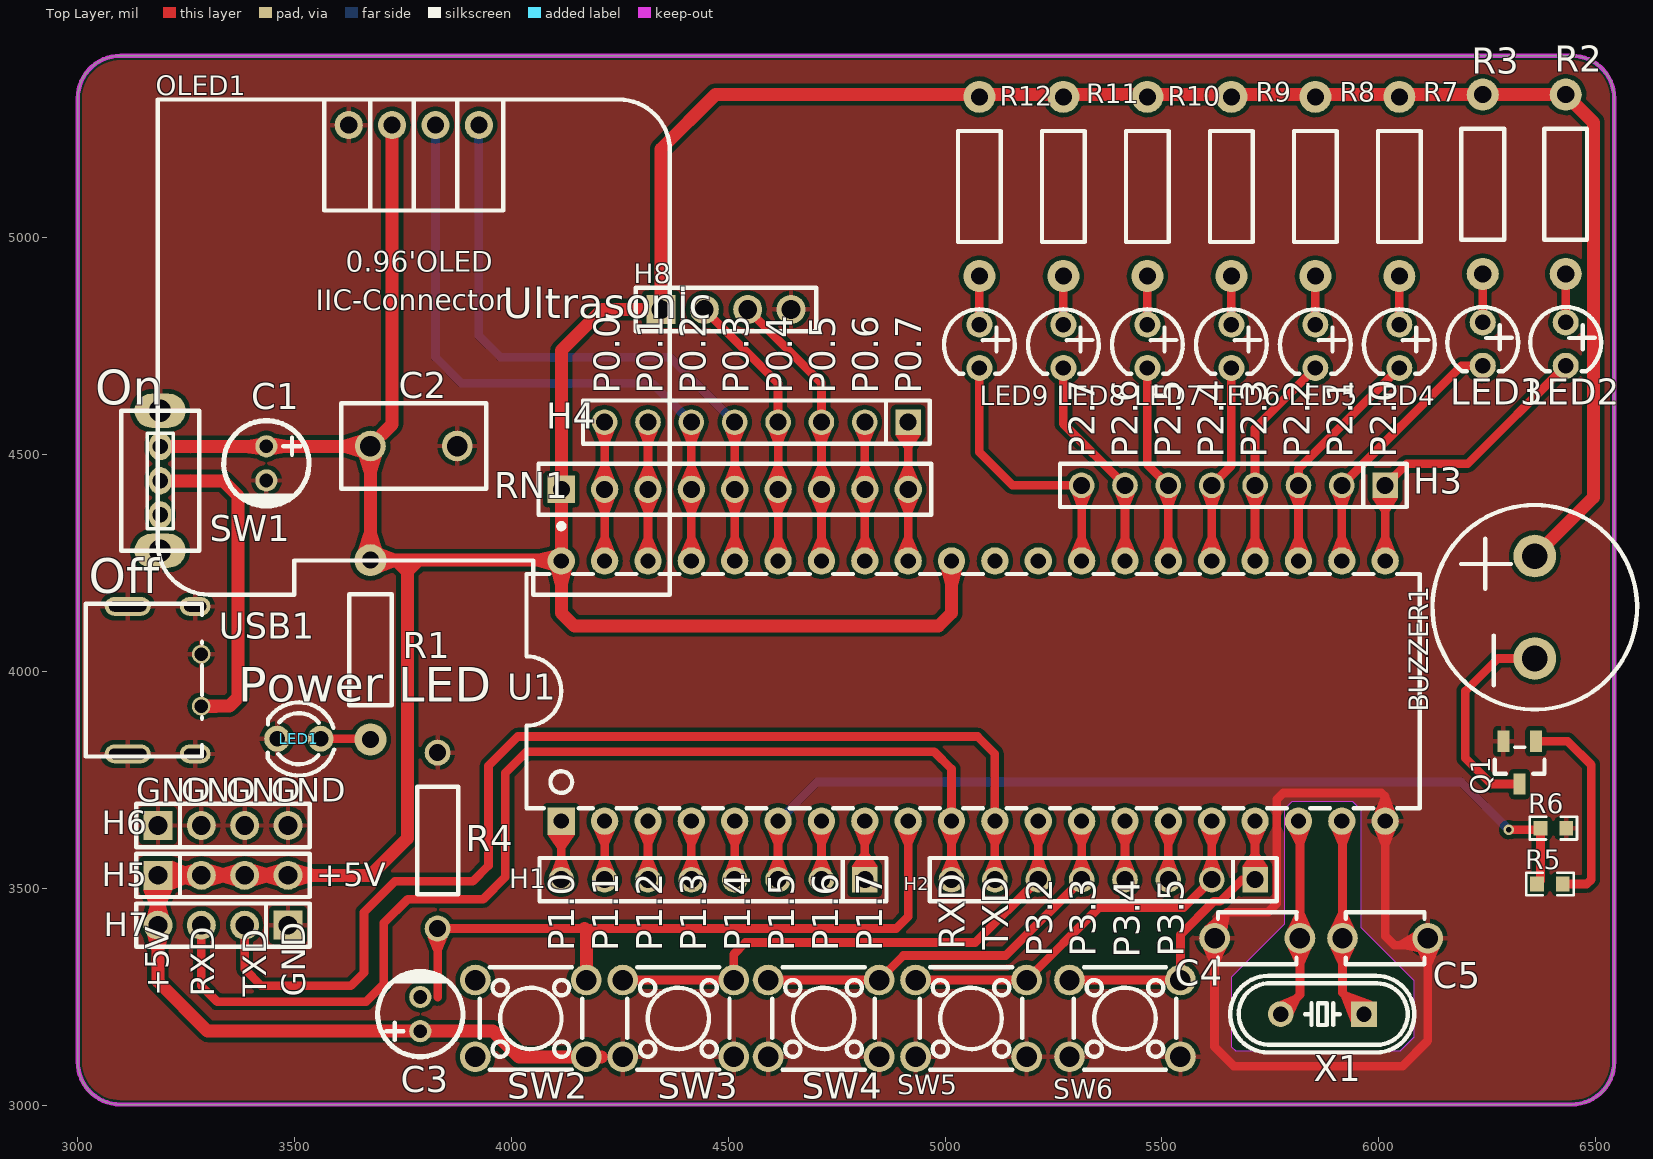
[diagram p0: Top Layer view]
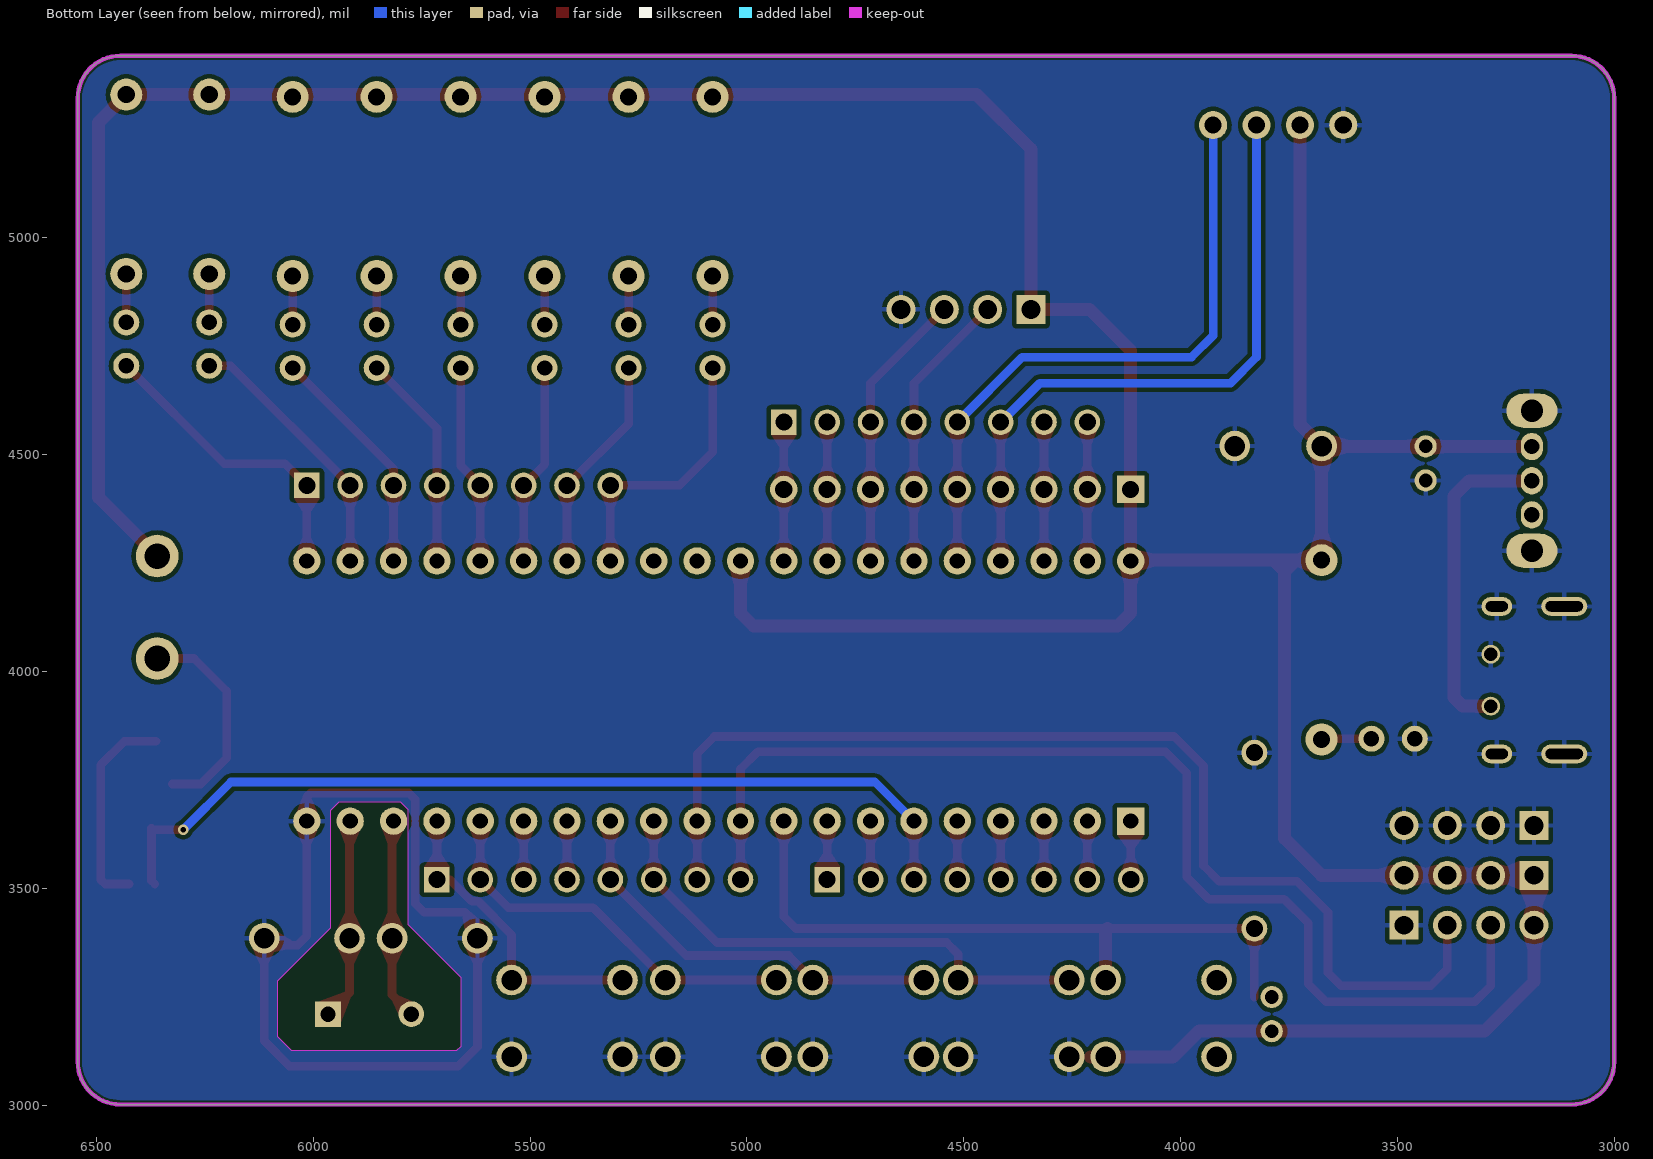
[diagram p1: Bottom Layer view, seen from below]
# Altium PCB MISC49889.pcbdoc
Units mil, origin at the board's own origin, x right, y up, seen from the top; angles counter-clockwise.
Board outline 3543.31 x 2418.5 mil, 2 copper layers (Top Layer, Bottom Layer), stack 62.206 mil thick; 47 components, 49 nets, 191 pads, 1 vias.

## Layer stack, top to bottom
Top Solder Mask Layer: solder mask 0.394, Dk 3.3
Top Layer: signal copper 1.379
Dielectric1: surface 59.449, FR4, Dk 4.5
Bottom Layer: signal copper 1.378
Bottom Solder Mask Layer: solder mask 0.394, Dk 3.3

## Board outline
3098.43,5420 ccw(c3098.43,5321.57) 3000,5321.57 3000,3099.92 ccw(c3098.43,3099.92) 3098.43,3001.5 6444.88,3001.5 ccw(c6444.88,3099.92) 6543.31,3099.92 6543.31,5321.57 ccw(c6444.88,5321.57) 6444.88,5420 3098.43,5420

## Design rules (kind name [scope] priority, off if disabled: settings)
BoardOutlineClearance copperThickness2oz_1 [All] p2 off: genericclearance=8 ignorepadtopadclearanceinfootprint=FALSE except(0: Arc-SplitContinuation Track-SplitContinuation SMDPad-SplitContinuation THPad-SplitContinuation Via-SplitContinuation Fill-SplitContinuation Region-SplitContinuation Poly-SplitContinuation Text-SplitContinuation Hole-SplitContinuation; 6: SMDPad-CutoutEdge THPad-CutoutEdge Via-CutoutEdge Fill-CutoutEdge Region-CutoutEdge Text-CutoutEdge Hole-CutoutEdge; 10: Poly-OutlineEdge Poly-CutoutEdge; 11.8: Arc-OutlineEdge Track-OutlineEdge SMDPad-OutlineEdge THPad-OutlineEdge Via-OutlineEdge Fill-OutlineEdge Region-OutlineEdge Text-OutlineEdge Hole-OutlineEdge Arc-CutoutEdge Track-CutoutEdge)
BoardOutlineClearance Plane_innerPlane_1 [All] p4 off: genericclearance=6 ignorepadtopadclearanceinfootprint=FALSE except(0: Arc-SplitContinuation Track-SplitContinuation SMDPad-SplitContinuation THPad-SplitContinuation Via-SplitContinuation Fill-SplitContinuation Region-SplitContinuation Poly-SplitContinuation Text-SplitContinuation Hole-SplitContinuation; 5.98: SMDPad-CutoutEdge THPad-CutoutEdge Via-CutoutEdge Fill-CutoutEdge Region-CutoutEdge Text-CutoutEdge Hole-CutoutEdge; 10: Poly-OutlineEdge Poly-CutoutEdge; 11.81: Arc-OutlineEdge Track-OutlineEdge SMDPad-OutlineEdge THPad-OutlineEdge Via-OutlineEdge Fill-OutlineEdge Region-OutlineEdge Text-OutlineEdge Hole-OutlineEdge Arc-CutoutEdge Track-CutoutEdge)
BoardOutlineClearance Copper_copperRegion_1 [All] p6 off: genericclearance=6 ignorepadtopadclearanceinfootprint=FALSE except(0: Arc-SplitContinuation Track-SplitContinuation SMDPad-SplitContinuation THPad-SplitContinuation Via-SplitContinuation Fill-SplitContinuation Region-SplitContinuation Poly-SplitContinuation Text-SplitContinuation Hole-SplitContinuation; 5.98: SMDPad-CutoutEdge THPad-CutoutEdge Via-CutoutEdge Fill-CutoutEdge Region-CutoutEdge Text-CutoutEdge Hole-CutoutEdge; 10: Poly-OutlineEdge Poly-CutoutEdge; 11.81: Arc-OutlineEdge Track-OutlineEdge SMDPad-OutlineEdge THPad-OutlineEdge Via-OutlineEdge Fill-OutlineEdge Region-OutlineEdge Text-OutlineEdge Hole-OutlineEdge Arc-CutoutEdge Track-CutoutEdge)
BoardOutlineClearance copperThickness1oz_1 [All] p8: genericclearance=6 ignorepadtopadclearanceinfootprint=FALSE except(0: Arc-SplitContinuation Track-SplitContinuation SMDPad-SplitContinuation THPad-SplitContinuation Via-SplitContinuation Fill-SplitContinuation Region-SplitContinuation Poly-SplitContinuation Text-SplitContinuation Hole-SplitContinuation; 5.98: SMDPad-CutoutEdge THPad-CutoutEdge Via-CutoutEdge Fill-CutoutEdge Region-CutoutEdge Text-CutoutEdge Hole-CutoutEdge; 10: Poly-OutlineEdge Poly-CutoutEdge; 11.81: Arc-OutlineEdge Track-OutlineEdge SMDPad-OutlineEdge THPad-OutlineEdge Via-OutlineEdge Fill-OutlineEdge Region-OutlineEdge Text-OutlineEdge Hole-OutlineEdge Arc-CutoutEdge Track-CutoutEdge)
Clearance copperThickness2oz [All] p1 off: gap=8 ignorepadtopadclearanceinfootprint=FALSE except(6: SMDPad-Track SMDPad-SMDPad THPad-Track SMDPad-THPad THPad-THPad Track-Via SMDPad-Via THPad-Via Via-Via Fill-Track Region-Track Fill-SMDPad Region-SMDPad Fill-THPad Region-THPad Fill-Via Region-Via Fill-Fill Fill-Region Region-Region Arc-Track Arc-SMDPad Arc-THPad Arc-Via Fill-Arc Region-Arc Arc-Arc Text-Track SMDPad-Text Text-THPad Text-Via Fill-Text Region-Text Arc-Text Text-Text Hole-Track Hole-SMDPad Hole-THPad Hole-Via Fill-Hole Region-Hole Hole-Arc Hole-Text; 10: Poly-Track Poly-SMDPad Poly-THPad Poly-Via Poly-Fill Poly-Region Poly-Poly Poly-Arc Poly-Text Poly-Hole)
Clearance Plane_innerPlane [All] p3 off: gap=6 ignorepadtopadclearanceinfootprint=FALSE except(5.98: SMDPad-Track SMDPad-SMDPad THPad-Track SMDPad-THPad THPad-THPad Track-Via SMDPad-Via THPad-Via Via-Via Fill-Track Region-Track Fill-SMDPad Region-SMDPad Fill-THPad Region-THPad Fill-Via Region-Via Fill-Fill Fill-Region Region-Region Arc-Track Arc-SMDPad Arc-THPad Arc-Via Fill-Arc Region-Arc Arc-Arc Text-Track SMDPad-Text Text-THPad Text-Via Fill-Text Region-Text Arc-Text Text-Text Hole-Track Hole-SMDPad Hole-THPad Hole-Via Fill-Hole Region-Hole Hole-Arc Hole-Text; 10: Poly-Track Poly-SMDPad Poly-THPad Poly-Via Poly-Fill Poly-Region Poly-Poly Poly-Arc Poly-Text Poly-Hole)
Clearance Copper_copperRegion [All] p5 off: gap=6 ignorepadtopadclearanceinfootprint=FALSE except(5.98: SMDPad-Track SMDPad-SMDPad THPad-Track SMDPad-THPad THPad-THPad Track-Via SMDPad-Via THPad-Via Via-Via Fill-Track Region-Track Fill-SMDPad Region-SMDPad Fill-THPad Region-THPad Fill-Via Region-Via Fill-Fill Fill-Region Region-Region Arc-Track Arc-SMDPad Arc-THPad Arc-Via Fill-Arc Region-Arc Arc-Arc Text-Track SMDPad-Text Text-THPad Text-Via Fill-Text Region-Text Arc-Text Text-Text Hole-Track Hole-SMDPad Hole-THPad Hole-Via Fill-Hole Region-Hole Hole-Arc Hole-Text; 10: Poly-Track Poly-SMDPad Poly-THPad Poly-Via Poly-Fill Poly-Region Poly-Poly Poly-Arc Poly-Text Poly-Hole)
Clearance copperThickness1oz [All] p7: gap=6 ignorepadtopadclearanceinfootprint=FALSE except(5.98: SMDPad-Track SMDPad-SMDPad THPad-Track SMDPad-THPad THPad-THPad Track-Via SMDPad-Via THPad-Via Via-Via Fill-Track Region-Track Fill-SMDPad Region-SMDPad Fill-THPad Region-THPad Fill-Via Region-Via Fill-Fill Fill-Region Region-Region Arc-Track Arc-SMDPad Arc-THPad Arc-Via Fill-Arc Region-Arc Arc-Arc Text-Track SMDPad-Text Text-THPad Text-Via Fill-Text Region-Text Arc-Text Text-Text Hole-Track Hole-SMDPad Hole-THPad Hole-Via Fill-Hole Region-Hole Hole-Arc Hole-Text; 10: Poly-Track Poly-SMDPad Poly-THPad Poly-Via Poly-Fill Poly-Region Poly-Poly Poly-Arc Poly-Text Poly-Hole)
DiffPairsRouting differentialPair [All] p1: maxlimit=6 minlimit=6 mostfreqgap=6 toplayer_minwidth=5 toplayer_prefwidth=10 toplayer_maxwidth=100 toplayer_mingap=6 toplayer_prefgap=6 toplayer_maxgap=6 bottomlayer_minwidth=5 bottomlayer_prefwidth=10 bottomlayer_maxwidth=100 bottomlayer_mingap=6 bottomlayer_prefgap=6 bottomlayer_maxgap=6 maxuncoupledlength=10
HoleToHoleClearance otherClearance [All] p1: gap=11.8 allowstackedmicrovias=TRUE
Length netLength [All] p1: minlimit=0 maxlimit=0
PasteMaskExpansion pasteMaskExpansion [All] p1: expansion=0
PlaneConnect innerPlane [All] p1: planeconnectstyle=Relief reliefexpansion=20 reliefentries=4 reliefconductorwidth=10 reliefairgap=10
PolygonConnect copperRegion [All] p1: connectstyle=Relief reliefconductorwidth=10 reliefentries=4 polygonreliefangle="90 Angle" airgapwidth=10 via.connectstyle=Relief via.reliefconductorwidth=10 via.reliefentries=4 via.polygonreliefangle="90 Angle" via.airgapwidth=10
RoutingVias viaSize [All] p1: holewidth=12 width=24 viastyle="Through Hole" minholewidth=11.8 minwidth=19.7 maxholewidth=248 maxwidth=393.7
SolderMaskExpansion solderMaskExpansion [IsVia] p1: expansion=-1000 istentingtop=TRUE
SolderMaskExpansion solderMaskExpansion [All] p2: expansion=2 istentingtop=FALSE
Width copperThickness2oz_2 [All] p1 off: maxlimit=100 minlimit=8 preferedwidth=10
Width copperThickness1oz_2 [All] p2: maxlimit=100 minlimit=5 preferedwidth=10

## Components (designator, comment, footprint, x,y, rotation, side; value= is the part's Value field where it differs from the comment)
BUZZER1 "buzzer" BUZ-TH_BD12.0-P6.00-D0.9-RD 6360.02,4148.07 r90 top
C1 "10uF" CAP-TH_BD5.0-P2.00-D0.8-FD 3435,4480 r270 top
C2 "100nF" CAP-TH_L8.5-W5.0-P5.00-D1.2 3775,4520 r180 top
C3 "10uF" CAP-TH_BD5.0-P2.00-D0.8-FD 3790,3210 r90 top
C4 "47pF" CAP-TH_L4.5-W3.0-P5.00-D1.2 5720,3385 r0 top
C5 "47pF" CAP-TH_L4.5-W3.0-P5.00-D1.2 6015,3385 r180 top
H1 "" HDR-TH_8P-P2.54-V-M 4465,3520 r180 top
H2 "" HDR-TH_8P-P2.54-V-M 5365,3520 r180 top
H3 "" HDR-TH_8P-P2.54-V-M 5665,4429.22 r180 top
H4 "" HDR-TH_8P-P2.54-V-M 4565,4575 r180 top
H5 "" HDR-TH_4P-P2.54-V-M 3335,3530 r0 top
H6 "" HDR-TH_4P-P2.54-V-M 3335,3645 r0 top
H7 "" HDR-TH_4P-P2.54-V-M 3335,3415 r180 top
H8 "" HDR-TH_4P-P2.54-V-F 4495,4835 r0 top
LED1 "204-10SURD/S530-A3-L" LED-TH_BD3.0-P2.54-FD 3510,3845 r180 top
LED2 "204-10SYGD/S530-E3" LED-TH_BD3.8-P2.54-FD 6431.32,4755 r270 top
LED3 "204-10SYGD/S530-E3" LED-TH_BD3.8-P2.54-FD 6240,4755 r270 top
LED4 "204-10SYGD/S530-E3" LED-TH_BD3.8-P2.54-FD 6047.65,4750 r270 top
LED5 "204-10SYGD/S530-E3" LED-TH_BD3.8-P2.54-FD 5853.97,4750 r270 top
LED6 "204-10SYGD/S530-E3" LED-TH_BD3.8-P2.54-FD 5660.3,4750 r270 top
LED7 "204-10SYGD/S530-E3" LED-TH_BD3.8-P2.54-FD 5466.62,4750 r270 top
LED8 "204-10SYGD/S530-E3" LED-TH_BD3.8-P2.54-FD 5272.95,4750 r270 top
LED9 "204-10SYGD/S530-E3" LED-TH_BD3.8-P2.54-FD 5079.27,4750 r270 top
OLED1 "" 0.96OLED_4P 3775,5260 r0 top
Q1 "" S8550P_SOT 6325.02,3787.99 r90 top
R1 "1kΩ" RES-TH_BD2.5-L6.5-P10.50-D0.6 3675,4050 r270 top
R2 "1kΩ" RES-TH_BD2.5-L6.5-P10.50-D0.6 6431.32,5123.52 r270 top
R3 "1kΩ" RES-TH_BD2.5-L6.5-P10.50-D0.6 6240,5123.52 r270 top
R4 "10kΩ" RES-TH_BD2.4-L6.3-P10.30-D0.6 3830,3610 r270 top
R5 "1K" R0603 6395,3510 r0 top
R6 "1K" R0603 6402.72,3638.61 r0 top
R7 "1kΩ" RES-TH_BD2.5-L6.5-P10.50-D0.6 6047.65,5118.52 r270 top
R8 "1kΩ" RES-TH_BD2.5-L6.5-P10.50-D0.6 5853.97,5118.52 r270 top
R9 "1kΩ" RES-TH_BD2.5-L6.5-P10.50-D0.6 5660.3,5118.52 r270 top
R10 "1kΩ" RES-TH_BD2.5-L6.5-P10.50-D0.6 5466.62,5118.52 r270 top
R11 "1kΩ" RES-TH_BD2.5-L6.5-P10.50-D0.6 5272.95,5118.52 r270 top
R12 "1kΩ" RES-TH_BD2.5-L6.5-P10.50-D0.6 5079.27,5118.52 r270 top
RN1 "10kΩ" RES-ARRAY-TH_9P-P2.54-D1.0 4515.15,4420.16 r0 top
SW1 "SS-12D02-VG4" SW-TH_SS-12D02-VG4 3190,4440 r90 top
SW2 "" SW-TH_4P-L6.0-W6.0-P4.50-LS6.5 4045,3200 r180 top
SW3 "" SW-TH_4P-L6.0-W6.0-P4.50-LS6.5 4385,3200 r0 top
SW4 "" SW-TH_4P-L6.0-W6.0-P4.50-LS6.5 4720,3200 r0 top
SW5 "" SW-TH_4P-L6.0-W6.0-P4.50-LS6.5 5060,3200 r0 top
SW6 "" SW-TH_4P-L6.0-W6.0-P4.50-LS6.5 5415,3200 r0 top
U1 "STC89C52RC-40I-PDIP40" DIP-40_L52.0-W13.7-P2.54-LS15.2-BL 5065,3955 r0 top
USB1 "TYPE-C-31-M-33" USB-C-TH_TYPE-C-31-M-33 3200,3980 r270 top
X1 "11.0592MHz" HC-49US_L11.5-W4.5-P4.88 5870,3210 r180 top

## Footprints (in the part's own frame and the unit in brackets; to place one, negate y for a bottom-side part, rotate by r counter-clockwise, add the part's x,y. Pads: shape width x height; smd on the part's side, far side on the other; paste and mask are expansions set on the pad)
0.96OLED_4P [mm]
  round 1.65 hole 1 copper offset 0,0: 1(-3.81,-0.001) 2(-1.27,0.002) 3(1.27,0.002) 4(3.81,0.002)
  silkscreen extent -15,-27.5 15,1.5
BUZ-TH_BD12.0-P6.00-D0.9-RD [mm]
  round 2.5 hole 1.5 paste+0 mask+0.05: 1(-3,0) 2(3,0)
  silkscreen extent -5.99,-5.99 5.99,5.99
CAP-TH_BD5.0-P2.00-D0.8-FD [mm]
  round 1.3 hole 0.8 paste+0 mask+0.051: 1(-1,0) 2(1,0)
  silkscreen extent -2.5,-2.5 2.5,2.5
CAP-TH_L4.5-W3.0-P5.00-D1.2 [mm]
  round 1.8 hole 1.2 paste+0 mask+0.051: 1(-2.5,0) 2(2.5,0)
  silkscreen extent -2.3,-1.52 2.31,1.52
CAP-TH_L8.5-W5.0-P5.00-D1.2 [mm]
  round 1.8 hole 1.2 paste+0 mask+0.051: 1(-2.54,0) 2(2.54,0)
  silkscreen extent -4.25,-2.5 4.25,2.5
DIP-40_L52.0-W13.7-P2.54-LS15.2-BL [mil]
  rect 63x63 hole 35 paste+0 mask+2: 1(-950,-300)
  round 63 hole 35 paste+0 mask+2: 2(-850,-300) 3(-750,-300) 4(-650,-300) 5(-550,-300) 6(-450,-300) 7(-350,-300) 8(-250,-300) 9(-150,-300) 10(-50,-300) 11(50,-300) 12(150,-300) 13(250,-300) 14(350,-300) 15(450,-300) 16(550,-300) 17(650,-300) 18(750,-300) 19(850,-300) 20(950,-300) 21(950,300) 22(850,300) 23(750,300) 24(650,300) 25(550,300) 26(450,300) 27(350,300) 28(250,300) 29(150,300) 30(50,300) 31(-50,300) 32(-150,300) 33(-250,300) 34(-350,300) 35(-450,300) 36(-550,300) 37(-650,300) 38(-750,300) 39(-850,300) 40(-950,300)
  silkscreen extent -1030,-270 1030,270
HC-49US_L11.5-W4.5-P4.88 [mm]
  rect 1.5x1.5 hole 0.9 paste+0 mask+0.051: 1(-2.44,0)
  round 1.5 hole 0.9 paste+0 mask+0.051: 2(2.44,0)
  silkscreen extent -5.39,-2.25 5.39,2.25
HDR-TH_4P-P2.54-V-F [mm]
  rect 1.7x1.7 hole 1.1: 1(-3.81,0)
  round 1.7 hole 1.1: 2(-1.27,0) 3(1.27,0) 4(3.81,0)
  silkscreen extent -5.29,-1.27 5.29,1.27
HDR-TH_4P-P2.54-V-M [mm]
  rect 1.7x1.7 hole 1.1 paste+0 mask+0.051: 1(-3.81,0)
  round 1.7 hole 1.1 paste+0 mask+0.051: 2(-1.27,0) 3(1.27,0) 4(3.81,0)
  silkscreen extent -5.08,-1.27 5.08,1.27
HDR-TH_8P-P2.54-V-M [mm]
  rect 1.5x1.5 hole 1 paste+0 mask+0.051: 1(-8.89,0)
  round 1.5 hole 1 paste+0 mask+0.051: 2(-6.35,0) 3(-3.81,0) 4(-1.27,0) 5(1.27,0) 6(3.81,0) 7(6.35,0) 8(8.89,0)
  silkscreen extent -10.16,-1.27 10.16,1.27
LED-TH_BD3.0-P2.54-FD [mil]
  round 60 hole 36 paste+0 mask+2: 1(-50,0) 2(50,0)
  silkscreen extent -81,-84 72,85
LED-TH_BD3.8-P2.54-FD [mil]
  round 60 hole 35.43 paste+0 mask+2: 1(-50,0) 2(50,0)
  silkscreen extent -85,-82 63,82
R0603 [mil]
  rect 31.75x34.02 smd paste-3937.01 mask+2: 1(-29.66,0) 2(29.66,0)
  silkscreen extent -55,-26 55,26
RES-ARRAY-TH_9P-P2.54-D1.0 [mm]
  rect 1.6x1.6 hole 1 paste+0 mask+0.051: 1(-10.16,0)
  round 1.6 hole 1 paste+0 mask+0.051: 2(-7.62,0) 3(-5.08,0) 4(-2.54,0) 5(0,0) 6(2.54,0) 7(5.08,0) 8(7.62,0) 9(10.16,0)
  silkscreen extent -11.5,-2.31 11.5,1.5
RES-TH_BD2.4-L6.3-P10.30-D0.6 [mil]
  round 60 hole 39.37 paste+0 mask+2: 1(-202.76,0) 2(202.76,0)
  silkscreen extent -124,-47 124,47
RES-TH_BD2.5-L6.5-P10.50-D0.6 [mil]
  round 74 hole 39.37 paste+0 mask+2: 1(-206.69,0) 2(206.69,0)
  silkscreen extent -128,-49 128,49
S8550P_SOT [mil]
  rect 49.2x27.6 smd paste+0 mask+2: 1(50.84,-37.4) 2(50.84,37.4) 3(-47.56,0)
  silkscreen extent -24,-58 37,58
SW-TH_4P-L6.0-W6.0-P4.50-LS6.5 [mm]
  round 1.8 hole 1.2 paste+0 mask+0.051: 1(-3.25,2.25) 2(3.25,2.25) 3(-3.25,-2.25) 4(3.25,-2.25)
  silkscreen extent -3,-3 3,3
SW-TH_SS-12D02-VG4 [mm]
  oval 1.6x1.3 hole 0.9 paste+0 mask+0.051: 1(-2,0) 2(-0.007,0) 3(2,0)
  oval 2x3 hole 1.3 paste+0 mask+0.051: 4(4.1,0) 5(-4.1,0)
  silkscreen extent -4.1,-2.29 4.1,2.29
USB-C-TH_TYPE-C-31-M-33 [mm]
  oval 1.1x1.8 hole 0.6 slot 1.3 at 90 deg paste+0 mask+0.05: 3(4.32,1.8) 6(-4.32,1.8)
  oval 1.1x2.7 hole 0.6 slot 2.2 at 90 deg paste+0 mask+0.05: 4(4.32,-2.15) 5(-4.32,-2.15)
  round 1.1 hole 0.8 paste+0 mask+0.05: A9(1.52,2.15) B12(-1.52,2.15)
  silkscreen extent -4.47,-4.6 4.47,2.2

## Via types
v1: diameter 24, hole 12, Top Layer to Bottom Layer, 1 vias

## Nets (pads, with @x,y where several pads share a name; then routed paths per layer and width w, separated by ;. In a path a pad name is that pad's centre, name@x,y a point inside that pad or via, vN(x,y) a via of type N, cw(c..) or ccw(c..) an arc to the next point about the centre after c; other vN are vias at no path point)
$1N2977: LED1.1 R1.2 | length 120.7
  Top Layer w20: LED1.1 3678.31,3845 R1.2@3680,3843.31
$1N4098: LED2.1 R2.2 | length 111.8
  Top Layer w20: LED2.1 R2.2
$1N4101: LED3.1 R3.2 | length 111.8
  Top Layer w20: LED3.1 R3.2
$1N15801: Q1.1 R5.2 | length 484.4
  Top Layer w20: Q1.1 6436.17,3838.83 6490,3785 6490,3520 6480,3510 R5.2
$1N15923: BUZZER1.1 Q1.3 | length 495.8
  Top Layer w20: Q1.3 6259.57,3740.43 6200,3800 6200,3955 6274.96,4029.96 BUZZER1.1
$1N16102: LED5.1 R8.2 | length 111.8
  Top Layer w20: LED5.1 R8.2
$1N16108: LED4.1 R7.2 | length 111.8
  Top Layer w20: LED4.1 R7.2
$1N16243: LED7.1 R10.2 | length 111.8
  Top Layer w20: LED7.1 R10.2
$1N16249: LED6.1 R9.2 | length 111.8
  Top Layer w20: LED6.1 R9.2
$1N16384: LED9.1 R12.2 | length 111.8
  Top Layer w20: LED9.1 R12.2
$1N16390: LED8.1 R11.2 | length 111.8
  Top Layer w20: LED8.1 R11.2
+5V: BUZZER1.2 C1.1 C2.2 C3.1 H5.1 H5.2 H5.3 H5.4 H7.4 H8.1 OLED1.2 R1.1 R2.1 R3.1 R7.1 R8.1 R9.1 R10.1 R11.1 R12.1 RN1.1 SW1.3 SW2.1 SW2.2 U1.31 U1.40 | length 10189
  Top Layer w20: C1.1@3434.37,4518.74 C1.1 ; U1.40 U1.40@4115.15,4255.15
  Top Layer w30: SW1.3 C1.1@3434.37,4518.74 ; C1.1 3674.37,4519.37 C2.2 ; OLED1.2@3725,5260.05 3725,4570 C2.2 ; 3760,4256.65 3760,4230.64 ; U1.40 4115.15,4254.85 4115.15,4135 4145.15,4105 4985,4105 5015,4135 U1.31 ; SW2.1@4207.95,3111.42 4017.05,3111.42 3957.84,3170.63 C3.1 3299.37,3170.63 3185,3285 H7.4 H5.1 H5.2 H5.3 H5.4 3675,3530 3760,3615 3760,4230.64 ; BUZZER1.2 6495,4401.16 6495,5266.53 R2.1 R3.1 4470.21,5330.21 4345,5205 H8.1 4210,4835 4115.15,4740.15 RN1.1 4115.15,4255.15 4113.61,4256.69 3785.2,4256.69 ; C2.2 R1.1 3733.95,4256.69 ; 3733.95,4256.69 3760,4256.69 3785.2,4256.69 ; 3733.95,4256.69 3760,4230.64 ; 3760,4230.64 3785.2,4255.84 3785.2,4256.69
GND: C1.2 C2.1 C4.1 C5.1 H6.1 H6.2 H6.3 H6.4 H7.1 H8.4 LED1.2 OLED1.1 Q1.2 R4.1 R6.2 SW1.4 SW1.5 SW3.3 SW3.4 SW4.3 SW4.4 SW5.3 SW5.4 SW6.3 SW6.4 U1.20 USB1.3 USB1.4 USB1.5 USB1.6 USB1.B12 | length 2144.4
  Top Layer w20: C5.1 C5.1@6113.43,3369.09 ; C5.1@6113.43,3369.09 6113.43,3148.43 6055,3090 5666.57,3090 5621.57,3135 5621.57,3416.57 5650,3445 5745,3445 5765,3465 5765,3705 5780,3720 6006.04,3720 6015,3711.04 U1.20 6015,3390 6035.91,3369.09 C5.1@6113.43,3369.09
P0.0: H4.8 RN1.2 U1.39 | length 320.1
  Top Layer w20: U1.39 4215.15,4255.15 RN1.2 4215.15,4574.85 H4.8
P0.1: H4.7 RN1.3 U1.38 | length 320.1
  Top Layer w20: U1.38 4315.15,4255.15 RN1.3 4315.15,4574.85 H4.7
P0.2: H4.6 OLED1.3 RN1.4 U1.37 | length 1507.3
  Top Layer w20: U1.37 4415.15,4255.15 RN1.4 4415.15,4574.85 H4.6
  Bottom Layer w20: OLED1.3@3825,5260.05 3825,4725 3885,4665 4325,4665 H4.6
P0.3: H4.5 OLED1.4 RN1.5 U1.36 | length 1478
  Top Layer w20: U1.36 4515.15,4255.15 RN1.5 4515.15,4574.85 H4.5
  Bottom Layer w20: OLED1.4@3925,5260.05 3925,4775 3975,4725 4365,4725 H4.5
P0.4: H4.4 H8.2 RN1.6 U1.35 | length 650.5
  Top Layer w20: H8.2 4615,4665 H4.4 4615.15,4574.85 RN1.6 4615.15,4255.15 U1.35
P0.5: H4.3 H8.3 RN1.7 U1.34 | length 650.5
  Top Layer w20: H8.3 4715,4665 H4.3 4715.15,4574.85 RN1.7 4715.15,4255.15 U1.34
P0.6: H4.2 RN1.8 U1.33 | length 320.1
  Top Layer w20: U1.33 4815.15,4255.15 RN1.8 4815.15,4574.85 H4.2
P0.7: H4.1 RN1.9 U1.32 | length 320.1
  Top Layer w20: U1.32 4915,4420.01 RN1.9 4915,4420.31 H4.1
P1.0: H1.8 U1.1 | length 135
  Top Layer w20: H1.8 U1.1
P1.1: H1.7 U1.2 | length 135
  Top Layer w20: H1.7 U1.2
P1.2: H1.6 U1.3 | length 135
  Top Layer w20: H1.6 U1.3
P1.3: H1.5 U1.4 | length 135
  Top Layer w20: H1.5 U1.4
P1.4: H1.4 U1.5 | length 135
  Top Layer w20: H1.4 U1.5
P1.5: H1.3 R5.1 R6.1 U1.6 | length 2109.2
  Top Layer w20: H1.3 U1.6 ; v1(6300,3635) 6369.45,3635 R6.1 6373.06,3517.72 R5.1
  Bottom Layer w20: U1.6 4705,3745 6190,3745 v1(6300,3635)
P1.6: H1.2 U1.7 | length 135
  Top Layer w20: H1.2 U1.7
P1.7: H1.1 U1.8 | length 135
  Top Layer w20: H1.1 U1.8
P2.0: H3.1 LED2.2 U1.21 | length 704.8
  Top Layer w20: U1.21 H3.1 6064.52,4478.74 6205.07,4478.74 LED2.2
P2.1: H3.2 LED3.2 U1.22 | length 613.5
  Top Layer w20: U1.22 H3.2 6190.78,4705 LED3.2
P2.2: H3.3 LED4.2 U1.23 | length 541.4
  Top Layer w20: U1.23 H3.3 5815,4467.35 LED4.2
P2.3: H3.4 LED5.2 U1.24 | length 502.6
  Top Layer w20: U1.24 H3.4 5715,4561.03 LED5.2
P2.4: H3.5 LED6.2 U1.25 | length 463.8
  Top Layer w20: U1.25 H3.5 5660.3,4474.52 LED6.2
P2.5: H3.6 LED7.2 U1.26 | length 465
  Top Layer w20: LED7.2 5466.62,4477.59 H3.6 U1.26
P2.6: H3.7 LED8.2 U1.27 | length 503.8
  Top Layer w20: LED8.2 5272.95,4571.27 H3.7 U1.27
P2.7: H3.8 LED9.2 U1.28 | length 635.9
  Top Layer w20: LED9.2 5079.27,4505.73 5155.78,4429.22 H3.8 U1.28
P3.2: H2.6 SW3.1 SW3.2 U1.12 | length 1223.6
  Top Layer w20: SW3.1 SW3.2 4512.95,3347.95 4540,3375 5070,3375 H2.6 U1.12
P3.3: H2.5 SW4.1 SW4.2 U1.13 | length 953.8
  Top Layer w20: SW4.1 SW4.2 4904.37,3345 5140,3345 H2.5 U1.13
P3.4: H2.4 U1.14 | length 135
  Top Layer w20: H2.4 U1.14
P3.5: H2.3 U1.15 | length 135
  Top Layer w20: H2.3 U1.15
P3.6: H2.2 SW5.1 SW5.2 U1.16 | length 913.8
  Top Layer w20: SW5.1 SW5.2 5354.37,3455 5550,3455 H2.2 U1.16
P3.7: H2.1 SW6.1 SW6.2 U1.17 | length 719.9
  Top Layer w20: SW6.1 SW6.2 5542.95,3392.95 5620,3470 5635,3470 5685,3520 H2.1 U1.17
RST: C3.2 R4.2 SW2.3 SW2.4 U1.9 | length 1594.9
  Top Layer w20: 3830,3249.37 R4.2 4168.45,3407.24 4887.24,3407.24 4915,3435 U1.9
  Top Layer w30: 4168.45,3407.24 4172.95,3402.74 SW2.3
RXD: H2.8 H7.3 U1.10 | length 2618.5
  Top Layer w20: H7.3 3285,3275 3321.61,3238.39 3664.91,3238.39 3706,3279.49 3706,3420 3761,3475 3935,3475 3986,3526 3986,3766 4035,3815 4975,3815 5015,3775 U1.10 H2.8
TXD: H2.7 H7.2 U1.11 | length 2608.5
  Top Layer w20: H7.2 3385,3313.93 3423.93,3275 3629.75,3275 3660,3305.25 3660,3445 3731,3516 3911,3516 3947.46,3552.46 3947.46,3782.46 4015,3850 5075,3850 5115,3810 U1.11 H2.7
VCC: SW1.2 USB1.A9 | length 752.5
  Top Layer w30: SW1.2 3335.02,4439.74 3370,4404.76 3370,3940.5 3349.65,3920.15 USB1.A9
X1: C5.2 U1.19 X1.1 | length 466.1
  Top Layer w20: U1.19 5916.57,3653.43 C5.2 5916.57,3259.49 X1.1
X2: C4.2 U1.18 X1.2 | length 464.8
  Top Layer w20: X1.2 5818.43,3254.49 C4.2 5818.43,3651.57 U1.18
pads on no net: SW1.1 U1.29 U1.30

## Polygon pours and split planes (outlines as drawn)
GND on Top Layer (solid, remove dead copper, pour order 0): 3000,5425 3000,3000 6545,3000 6545,5425
GND on Bottom Layer (solid, remove dead copper, pour order 2): 3000,5450 3000,3000 6545,3000 6545,5450

## Keep-outs
Board Outline Layer:
  region: 5799.4,3700 5781.9,3682.5 5781.9,3416.9 5660,3295 5660,3135 5670,3125 6050,3125 6082.3,3157.3 6082.3,3286.52 5960,3408.83 5960,3680 5940,3700
  lines w10: 3000,3099.92 3000,5321.57 cw(c3098.43,5321.57) 3098.43,5420 6444.88,5420 cw(c6444.88,5321.57) 6543.31,5321.57 6543.31,3099.92 cw(c6444.88,3099.92) 6444.88,3001.5 3098.43,3001.5 cw(c3098.43,3099.92) 3000,3099.92

## Other copper
Top Layer:
  region net +5V: 4991.38,4234.16 5000,4201.45 5030,4201.45 5038.62,4234.16
  region net P0.7: 4938.62,4275.84 4925,4308.55 4905,4308.55 4891.38,4275.84
  region net P0.6: 4838.72,4275.72 4825.15,4308.5 4805.15,4308.6 4791.47,4275.95
  region net P2.7: 5338.62,4275.84 5325,4308.55 5305,4308.55 5291.38,4275.84
  region net P0.5: 4738.72,4275.72 4725.15,4308.5 4705.15,4308.6 4691.47,4275.95
  region net P2.6: 5438.62,4275.84 5425,4308.55 5405,4308.55 5391.38,4275.84
  region net P0.4: 4638.72,4275.72 4625.15,4308.5 4605.15,4308.6 4591.47,4275.95
  region net P2.5: 5538.62,4275.84 5525,4308.55 5505,4308.55 5491.38,4275.84
  region net P2.4: 5638.62,4275.84 5625,4308.55 5605,4308.55 5591.38,4275.84
  region net P2.3: 5738.62,4275.84 5725,4308.55 5705,4308.55 5691.38,4275.84
  region net P0.3: 4538.72,4275.72 4525.15,4308.5 4505.15,4308.6 4491.47,4275.95
  region net P0.2: 4438.72,4275.72 4425.15,4308.5 4405.15,4308.6 4391.47,4275.95
  region net P2.2: 5838.62,4275.84 5825,4308.55 5805,4308.55 5791.38,4275.84
  region net P2.1: 5938.62,4275.84 5925,4308.55 5905,4308.55 5891.38,4275.84
  region net P2.0: 6038.62,4275.84 6025,4308.55 6005,4308.55 5991.38,4275.84
  region net P0.1: 4338.72,4275.72 4325.15,4308.5 4305.15,4308.6 4291.47,4275.95
  region net P0.0: 4238.72,4275.72 4225.15,4308.5 4205.15,4308.6 4191.47,4275.95
  region net +5V: 4095.46,4279.71 4062.27,4271.69 4060.66,4241.69 4092.93,4232.53
  region net +5V: 4091.47,4234.05 4100.15,4201.38 4130.15,4201.52 4138.72,4234.28
  region net RXD: 4991.38,3634.16 5005,3601.45 5025,3601.45 5038.62,3634.16
  region net P1.0: 4105,3593.5 4125,3593.5 4146.5,3623.5 4083.5,3623.5
  region net P1.1: 4191.38,3634.16 4205,3601.45 4225,3601.45 4238.62,3634.16
  region net P1.2: 4291.38,3634.16 4305,3601.45 4325,3601.45 4338.62,3634.16
  region net P1.3: 4391.38,3634.16 4405,3601.45 4425,3601.45 4438.62,3634.16
  region net P1.4: 4491.38,3634.16 4505,3601.45 4525,3601.45 4538.62,3634.16
  region net P1.5: 4591.38,3634.16 4605,3601.45 4625,3601.45 4638.62,3634.16
  region net P1.6: 4691.38,3634.16 4705,3601.45 4725,3601.45 4738.62,3634.16
  region net P1.7: 4791.38,3634.16 4805,3601.45 4825,3601.45 4838.62,3634.16
  region net RST: 4891.38,3634.16 4905,3601.45 4925,3601.45 4938.62,3634.16
  region net TXD: 5091.38,3634.16 5105,3601.45 5125,3601.45 5138.62,3634.16
  region net P3.2: 5191.38,3634.16 5205,3601.45 5225,3601.45 5238.62,3634.16
  region net P3.3: 5291.38,3634.16 5305,3601.45 5325,3601.45 5338.62,3634.16
  region net P3.4: 5391.38,3634.16 5405,3601.45 5425,3601.45 5438.62,3634.16
  region net P3.5: 5491.38,3634.16 5505,3601.45 5525,3601.45 5538.62,3634.16
  region net P3.6: 5591.38,3634.16 5605,3601.45 5625,3601.45 5638.62,3634.16
  region net P3.7: 5691.38,3634.16 5705,3601.45 5725,3601.45 5738.62,3634.16
  region net X2: 5793.78,3631.72 5808.43,3600.41 5828.43,3602.6 5840.75,3636.86
  region net X1: 5892.45,3633.01 5906.57,3600.96 5926.57,3601.96 5939.64,3635.37
  region net GND: 5991.38,3634.16 6005,3601.45 6025,3601.45 6038.62,3634.16
  region net GND: 6038.62,3675.84 6025,3708.55 6005,3708.55 5991.38,3675.84
  region net P0.0: 4238.77,4440.99 4225.15,4473.71 4205.15,4473.71 4191.53,4440.99
  region net P0.0: 4191.53,4399.33 4205.15,4366.62 4225.15,4366.62 4238.77,4399.33
  region net P0.1: 4338.77,4440.99 4325.15,4473.71 4305.15,4473.71 4291.53,4440.99
  region net P0.1: 4291.53,4399.33 4305.15,4366.62 4325.15,4366.62 4338.77,4399.33
  region net P0.2: 4438.77,4440.99 4425.15,4473.71 4405.15,4473.71 4391.53,4440.99
  region net P0.2: 4391.53,4399.33 4405.15,4366.62 4425.15,4366.62 4438.77,4399.33
  region net P0.3: 4538.77,4440.99 4525.15,4473.71 4505.15,4473.71 4491.53,4440.99
  region net P0.3: 4491.53,4399.33 4505.15,4366.62 4525.15,4366.62 4538.77,4399.33
  region net P0.4: 4638.77,4440.99 4625.15,4473.71 4605.15,4473.71 4591.53,4440.99
  region net P0.4: 4591.53,4399.33 4605.15,4366.62 4625.15,4366.62 4638.77,4399.33
  region net P0.5: 4738.77,4440.99 4725.15,4473.71 4705.15,4473.71 4691.53,4440.99
  region net P0.5: 4691.53,4399.33 4705.15,4366.62 4725.15,4366.62 4738.77,4399.33
  region net P0.6: 4838.77,4440.99 4825.15,4473.71 4805.15,4473.71 4791.53,4440.99
  region net P0.6: 4791.53,4399.33 4805.15,4366.62 4825.15,4366.62 4838.77,4399.33
  region net P0.7: 4938.67,4441.11 4925,4473.75 4905,4473.66 4891.43,4440.88
  region net P0.7: 4891.43,4399.44 4905,4366.67 4925,4366.57 4938.67,4399.22
  region net VCC: 3298.97,3903.91 3321.46,3905.15 3321.46,3935.15 3298.97,3936.39
  region net +5V: 3258.92,4533.74 3215.59,4524.65 3215.59,4512.84 3258.92,4503.74
  region net VCC: 3258.92,4424.74 3258.92,4454.74 3215.59,4445.65 3215.59,4433.84
  region net +5V: 3417.61,4538.14 3391.13,4533.74 3391.87,4503.74 3418.55,4499.77
  region net +5V: 3451.93,4500.18 3478.5,4504.37 3478.5,4534.37 3451.93,4538.56
  region net +5V: 3699.47,4228.94 3733.95,4241.69 3733.95,4271.69 3699.47,4284.44
  region net +5V: 3702.75,4281.16 3690,4319.59 3660,4319.59 3647.25,4281.16
  region net P1.7: 4805,3579.53 4785.47,3549.53 4844.53,3549.53 4825,3579.53
  region net P1.6: 4737.15,3539.53 4725,3570.2 4705,3570.2 4692.85,3539.53
  region net P1.5: 4637.15,3539.53 4625,3570.2 4605,3570.2 4592.85,3539.53
  region net P1.4: 4537.15,3539.53 4525,3570.2 4505,3570.2 4492.85,3539.53
  region net P1.3: 4437.15,3539.53 4425,3570.2 4405,3570.2 4392.85,3539.53
  region net P1.2: 4337.15,3539.53 4325,3570.2 4305,3570.2 4292.85,3539.53
  region net P1.1: 4237.15,3539.53 4225,3570.2 4205,3570.2 4192.85,3539.53
  region net P1.0: 4137.15,3539.53 4125,3570.2 4105,3570.2 4092.85,3539.53
  region net P3.7: 5705,3579.53 5685.47,3549.53 5744.53,3549.53 5725,3579.53
  region net P3.6: 5637.15,3539.53 5625,3570.2 5605,3570.2 5592.85,3539.53
  region net P3.5: 5537.15,3539.53 5525,3570.2 5505,3570.2 5492.85,3539.53
  region net P3.4: 5437.15,3539.53 5425,3570.2 5405,3570.2 5392.85,3539.53
  region net P3.3: 5337.15,3539.53 5325,3570.2 5305,3570.2 5292.85,3539.53
  region net P3.2: 5237.15,3539.53 5225,3570.2 5205,3570.2 5192.85,3539.53
  region net TXD: 5137.15,3539.53 5125,3570.2 5105,3570.2 5092.85,3539.53
  region net RXD: 5037.15,3539.53 5025,3570.2 5005,3570.2 4992.85,3539.53
  region net P2.0: 6005,4369.69 6025,4369.69 6044.53,4399.69 5985.47,4399.69
  region net P2.1: 5892.85,4409.69 5905,4379.02 5925,4379.02 5937.15,4409.69
  region net P2.2: 5792.85,4409.69 5805,4379.02 5825,4379.02 5837.15,4409.69
  region net P2.3: 5692.85,4409.69 5705,4379.02 5725,4379.02 5737.15,4409.69
  region net P2.4: 5592.85,4409.69 5605,4379.02 5625,4379.02 5637.15,4409.69
  region net P2.5: 5492.85,4409.69 5505,4379.02 5525,4379.02 5537.15,4409.69
  region net P2.6: 5392.85,4409.69 5405,4379.02 5425,4379.02 5437.15,4409.69
  region net P2.7: 5292.85,4409.69 5305,4379.02 5325,4379.02 5337.15,4409.69
  region net P0.7: 4925,4515.47 4944.53,4545.47 4885.47,4545.47 4905,4515.47
  region net P0.6: 4792.95,4555.36 4805.15,4524.75 4825.15,4524.85 4837.24,4555.58
  region net P0.5: 4692.95,4555.36 4705.15,4524.75 4725.15,4524.85 4737.24,4555.58
  region net P0.4: 4592.95,4555.36 4605.15,4524.75 4625.15,4524.85 4637.24,4555.58
  region net P0.3: 4492.95,4555.36 4505.15,4524.75 4525.15,4524.85 4537.24,4555.58
  region net P0.2: 4392.95,4555.36 4405.15,4524.75 4425.15,4524.85 4437.24,4555.58
  region net P0.1: 4292.95,4555.36 4305.15,4524.75 4325.15,4524.85 4337.24,4555.58
  region net P0.0: 4192.95,4555.36 4205.15,4524.75 4225.15,4524.85 4237.24,4555.58
  region net +5V: 3159.9,3392.87 3170,3358.11 3200,3358.11 3210.1,3392.87
  region net +5V: 3210.1,3437.13 3200,3471.89 3170,3471.89 3159.9,3437.13
  region net +5V: 3170,3451.54 3200,3451.54 3218.46,3496.54 3151.54,3496.54
  region net +5V: 3263.46,3545 3218.46,3563.46 3218.46,3496.54 3263.46,3515
  region net +5V: 3307.13,3504.9 3341.89,3515 3341.89,3545 3307.13,3555.1
  region net +5V: 3262.87,3555.1 3228.11,3545 3228.11,3515 3262.87,3504.9
  region net +5V: 3362.87,3555.1 3328.11,3545 3328.11,3515 3362.87,3504.9
  region net +5V: 3407.13,3504.9 3441.89,3515 3441.89,3545 3407.13,3555.1
  region net +5V: 3507.13,3504.9 3541.89,3515 3541.89,3545 3507.13,3555.1
  region net +5V: 3462.87,3555.1 3428.11,3545 3428.11,3515 3462.87,3504.9
  region net +5V: 3651.09,4546.15 3614.5,4534.37 3615.03,4504.37 3652.04,4493.01
  region net +5V: 3648.43,4496.56 3660,4459.76 3690,4459.76 3701.57,4496.56
  region net GND: 5650.43,3405.56 5657.07,3437.93 5635.02,3444.16 5597.57,3411.06
  region net GND: 5595,3361.56 5611.57,3324.76 5631.57,3324.76 5648.15,3361.56
  region net X2: 5791.85,3361.56 5808.43,3324.76 5828.43,3324.76 5845,3361.56
  region net X2: 5845,3408.44 5828.43,3445.24 5808.43,3445.24 5791.85,3408.44
  region net GND: 6086.85,3361.56 6103.43,3324.76 6123.43,3324.76 6140,3361.56
  region net GND: 6080.55,3398.22 6048.98,3379.09 6059.03,3359.09 6104.42,3350.73
  region net X1: 5890,3361.56 5906.57,3324.76 5926.57,3324.76 5943.15,3361.56
  region net X1: 5943.15,3408.44 5926.57,3445.24 5906.57,3445.24 5890,3408.44
  region net X1: 5929.46,3260.74 5915.32,3246.6 5936.53,3190.03 5986.03,3239.53
  region net X2: 5803.41,3208.15 5816.51,3238.42 5802.36,3252.57 5772.09,3239.47
  region net RST: 3807.5,3387.4 3820,3356.24 3840,3356.24 3852.5,3387.4

## Silkscreen, mask and mechanical layers (free items; w line width, h text height)
Top Silkscreen Layer:
  text "Ultrasonic" at 3980,4815 h70
  text "P0.0" at 4250,4640 h60 r90
  text "P0.1" at 4349.29,4640 h60 r90
  text "P0.2" at 4448.57,4640 h60 r90
  text "P0.3" at 4547.86,4640 h60 r90
  text "P0.4" at 4647.14,4640 h60 r90
  text "P0.5" at 4746.43,4640 h60 r90
  text "P0.6" at 4845.71,4640 h60 r90
  text "P0.7" at 4945,4640 h60 r90
  text "On" at 3040,4615 h80
  text "P2.7" at 5345,4493.3 h60 r90
  text "P2.6" at 5444.29,4493.3 h60 r90
  text "P2.5" at 5543.57,4493.3 h60 r90
  text "P2.4" at 5642.86,4493.3 h60 r90
  text "P2.3" at 5742.14,4493.3 h60 r90
  text "P2.2" at 5841.43,4493.3 h60 r90
  text "P2.1" at 5940.71,4493.3 h60 r90
  text "P2.0" at 6040,4493.3 h60 r90
  text "Off" at 3025,4180 h80
  text "Power LED" at 3370,3930 h80
  text "GND" at 3135,3700 h55
  text "GND" at 3238.9,3700 h55
  text "GND" at 3342.8,3700 h55
  text "GND" at 3446.7,3700 h55
  text "+5V" at 3550,3505 h55
  text "RXD" at 5045,3358.4 h60 r90
  text "TXD" at 5146,3358.4 h60 r90
  text "P1.0" at 4145,3355 h60 r90
  text "P1.1" at 4246.43,3355 h60 r90
  text "P1.2" at 4347.86,3355 h60 r90
  text "P1.3" at 4449.29,3355 h60 r90
  text "P1.4" at 4550.71,3355 h60 r90
  text "P1.5" at 4652.14,3355 h60 r90
  text "P1.6" at 4753.57,3355 h60 r90
  text "P1.7" at 4855,3355 h60 r90
  text "P3.2" at 5247,3341.7 h60 r90
  text "P3.3" at 5348,3341.7 h60 r90
  text "P3.5" at 5550,3341.7 h60 r90
  text "P3.4" at 5449,3340 h60 r90
  text "+5V" at 3210,3251.4 h55 r90
  text "RXD" at 3315,3250 h55 r90
  text "TXD" at 3435,3250 h55 r90
  text "GND" at 3525,3250 h55 r90